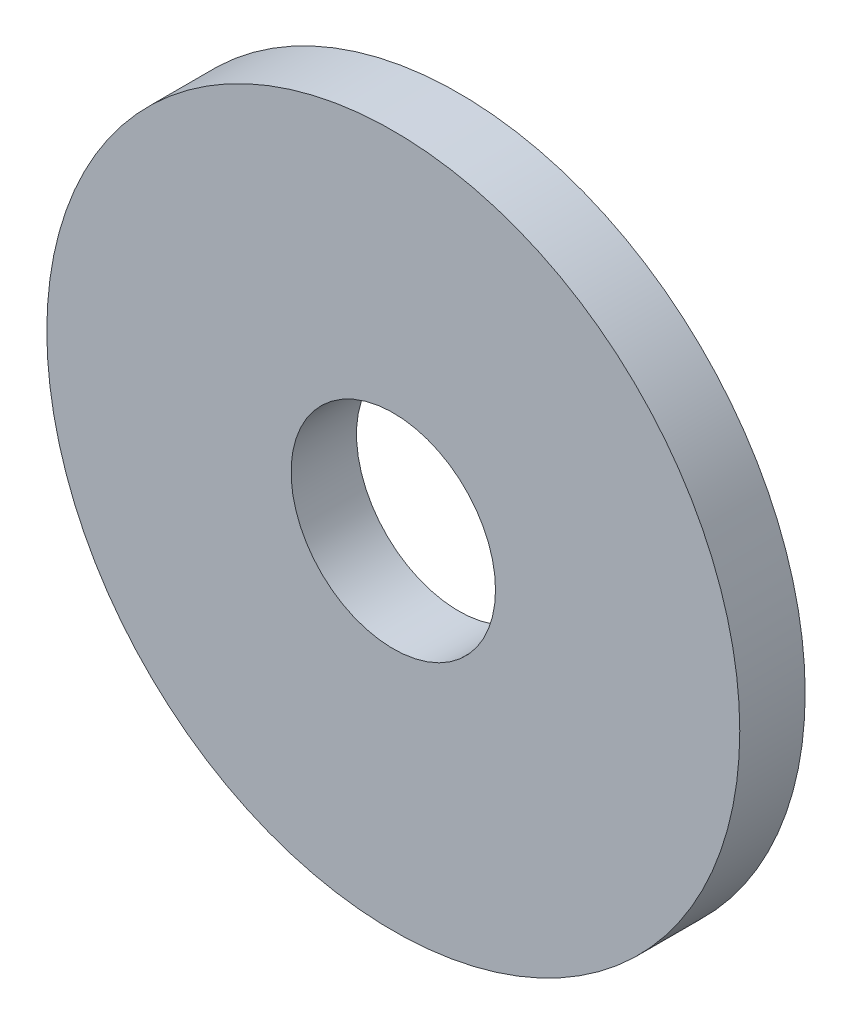
from build123d import *

# Parameters (mm, degrees)
SKETCH1_R           = 84.75
SKETCH1_R_2         = 25
BOSS_EXTRUDE1_DEPTH = 16


with BuildPart() as part:
    # Sketch1 → Boss-Extrude1 (new body)
    with BuildSketch(Plane.XY):
        Circle(SKETCH1_R)
        Circle(SKETCH1_R_2, mode=Mode.SUBTRACT)
    extrude(amount=BOSS_EXTRUDE1_DEPTH)


solid = part.part
